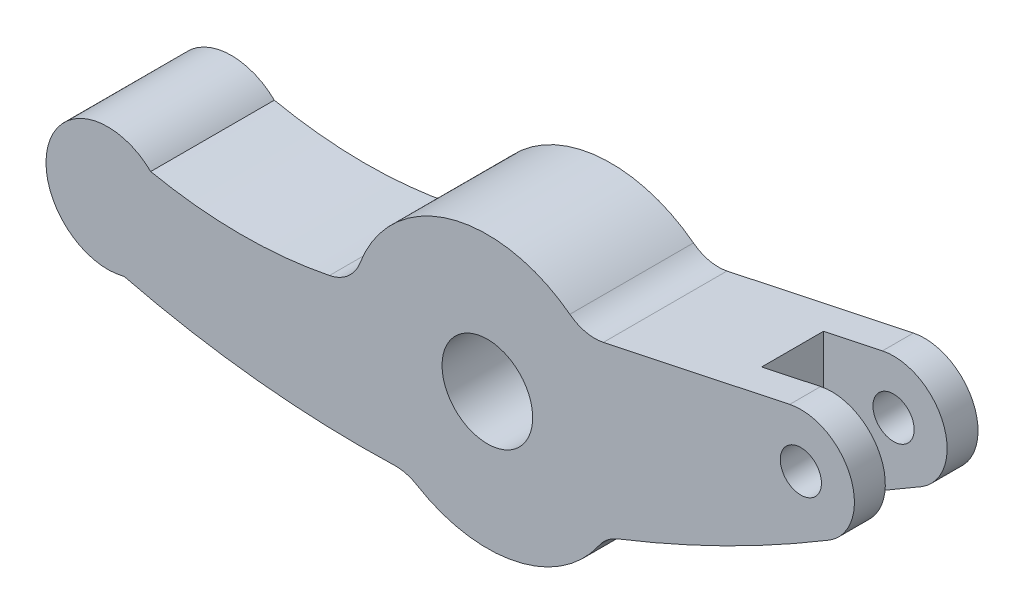
SolidWorks part; units mm, degrees
ref_plane "Front Plane" through (0, 0, 0) normal (0, 0, 1) x (1, 0, 0)
ref_plane "Top Plane" through (0, 0, 0) normal (0, 1, 0) x (1, 0, 0)
ref_plane "Right Plane" through (0, 0, 0) normal (1, 0, 0) x (0, 0, -1)
sketch "Sketch1" plane through (0, 0, 0) normal (0, 0, 1) x (1, 0, 0)
  line L7 (23.3648, -2.4326) -> (82.7627, 3.0066)
  line L8 (23.3729, -8.3627) -> (82.7596, -3.0293)
  arc A14 (23.3648, -2.4326) -> (23.3729, -8.3627) centre (8.6648, -5.4177) ccw
  arc A16 (82.7596, -3.0293) -> (82.7627, 3.0066) centre (100.5064, -0.0205) ccw
extrude "Boss-Extrude1" add sketch "Sketch1" along normal blind 10
sketch "Sketch7" plane through (0, 0, 0) normal (0, 0, -1) x (-1, 0, 0)
  circle A0 centre (-100.78, 0) radius 8
extrude "Cut-Extrude2" cut sketch "Sketch7" against normal blind 10
sketch "Sketch8" plane through (0, 0, 10) normal (0, 0, 1) x (1, 0, 0)
  circle A0 centre (8.6648, -5.4177) radius 6
extrude "Cut-Extrude3" cut sketch "Sketch8" against normal blind 14
sketch "Sketch17" plane through (0, 0, 0) normal (0, 0, -1) x (-1, 0, 0)
  line L1 (-115.8122, 9.3934) -> (-161.8976, 22.2751)
  line L2 (-118.4017, 1.9179) -> (-164.5896, 12.6443)
  arc A0 (-161.8976, 22.2751) -> (-164.5896, 12.6443) centre (-176.8637, 21.2668) ccw
  arc A1 (-118.4017, 1.9179) -> (-115.8122, 9.3934) centre (-100.78, 0) ccw
  circle A2 centre (-100.78, 0) radius 8
  arc A3 (-82.7627, 3.0066) -> (-82.7596, -3.0293) centre (-100.5064, -0.0205) ccw construction
  point P4 (-99.434, 4.8154)
  point P5 (-175.5177, 26.0822)
  point P6 (-102.126, -4.8154)
  point P7 (-178.2097, 16.4513)
extrude "Boss-Extrude2" add sketch "Sketch17" against normal blind 10
sketch "Sketch18" plane through (0, 0, 0) normal (0, 0, -1) x (-1, 0, 0)
  circle A0 centre (-176.8637, 21.2668) radius 6
extrude "Cut-Extrude10" cut sketch "Sketch18" against normal blind 10
sketch "Sketch20" plane through (0, 0, 10) normal (0, 0, 1) x (1, 0, 0)
  circle A0 centre (176.8637, 21.2668) radius 15
sketch "Sketch21" plane through (0, 0, 10) normal (0, 0, 1) x (1, 0, 0)
  circle A0 centre (8.6648, -5.4177) radius 15
sketch "Sketch22" plane through (0, 0, 10) normal (0, 0, 1) x (1, 0, 0)
  circle A0 centre (8.6648, -5.4177) radius 13
sketch "Sketch23" plane through (0, 0, 10) normal (0, 0, 1) x (1, 0, 0)
  line L0 (174.169, 33.9844) -> (97.0897, 17.6522)
  line L1 (181.1377, 8.9894) -> (108.1783, -16.4093)
  arc A0 (8.6648, -18.4177) -> (102.3485, -17.9315) centre (54.4178, 191.6593) ccw
  arc A3 (13.0493, 6.8206) -> (92.6784, 16.1882) centre (41.1609, 110.9854) ccw
  arc A6 (181.1377, 8.9894) -> (174.169, 33.9844) centre (176.8637, 21.2668) ccw
  arc A10 (13.0493, 6.8206) -> (8.6648, -18.4177) centre (8.6648, -5.4177) ccw
  arc A11 (102.3485, -17.9315) -> (108.1783, -16.4093) centre (100.78, 0) ccw
  arc A12 (92.6784, 16.1882) -> (97.0897, 17.6522) centre (100.5064, -0.0205) cw
extrude "Boss-Extrude3" add sketch "Sketch23" along normal blind 10
sketch "Sketch25" plane through (0, 0, 10) normal (0, 0, -1) x (-1, 0, 0)
  circle A0 centre (-8.6648, -5.4177) radius 5
extrude "Cut-Extrude11" cut sketch "Sketch25" against normal blind 20
sketch "Sketch26" plane through (0, 0, 20) normal (0, 0, 1) x (1, 0, 0)
  circle A0 centre (8.6648, -5.4177) radius 8.5
sketch "Sketch29" plane through (0, 0, 10) normal (0, 0, -1) x (-1, 0, 0)
  circle A0 centre (-176.8637, 21.2668) radius 5
extrude "Cut-Extrude12" cut sketch "Sketch29" against normal blind 10
sketch "Sketch30" plane through (0, 0, 0) normal (0, 0, -1) x (-1, 0, 0)
  line L2 (-181.1377, 8.9894) -> (-108.1783, -16.4093)
  line L3 (-97.0897, 17.6522) -> (-174.169, 33.9844)
  line L4 (-181.1377, 8.9894) -> (-108.1783, -16.4093)
  line L5 (-97.0897, 17.6522) -> (-174.169, 33.9844)
  arc A6 (-8.6648, -18.4177) -> (-13.0493, 6.8206) centre (-8.6648, -5.4177) ccw
  arc A7 (-102.3485, -17.9315) -> (-8.6648, -18.4177) centre (-54.4178, 191.6593) ccw
  arc A8 (-108.1783, -16.4093) -> (-102.3485, -17.9315) centre (-100.78, 0) ccw
  arc A9 (-174.169, 33.9844) -> (-181.1377, 8.9894) centre (-176.8637, 21.2668) ccw
  arc A10 (-92.6784, 16.1882) -> (-97.0897, 17.6522) centre (-100.5064, -0.0205) ccw
  arc A11 (-92.6784, 16.1882) -> (-13.0493, 6.8206) centre (-41.1609, 110.9854) ccw
  arc A12 (-8.6648, -18.4177) -> (-13.0493, 6.8206) centre (-8.6648, -5.4177) ccw
  arc A13 (-102.3485, -17.9315) -> (-8.6648, -18.4177) centre (-54.4178, 191.6593) ccw
  arc A14 (-108.1783, -16.4093) -> (-102.3485, -17.9315) centre (-100.78, 0) ccw
  arc A15 (-174.169, 33.9844) -> (-181.1377, 8.9894) centre (-176.8637, 21.2668) ccw
  arc A16 (-92.6784, 16.1882) -> (-97.0897, 17.6522) centre (-100.5064, -0.0205) ccw
  arc A17 (-92.6784, 16.1882) -> (-13.0493, 6.8206) centre (-41.1609, 110.9854) ccw
  dimension "D1" = 0
sketch "Sketch31" plane through (0, 0, 10) normal (0, 0, -1) x (-1, 0, 0)
  circle A0 centre (-100.78, 0) radius 11
extrude "Cut-Extrude13" cut sketch "Sketch31" against normal blind 10
extrude "Boss-Extrude5" add sketch "Sketch30" along normal blind 10 and the other way blind 10 contours L5 A15 L4 A14 A13 A12 A17 A16
sketch "Sketch32" plane through (0, 0, 10) normal (0, 0, 1) x (1, 0, 0)
  circle A0 centre (8.6648, -5.4177) radius 5
  circle A1 centre (100.78, 0) radius 11
  circle A2 centre (176.8637, 21.2668) radius 5
extrude "Cut-Extrude14" cut sketch "Sketch32" against normal blind 20
ref_plane "Plane1" through (0, 0, -2.5) normal (0, 0, -1) x (-1, 0, 0)
sketch "Sketch33" plane through (0, 0, -2.5) normal (0, 0, -1) x (-1, 0, 0)
  line L1 (-25.6648, -5.4177) -> (-25.6648, -33.5873)
  line L2 (-25.6648, -33.5873) -> (16.718, -33.5873)
  line L3 (16.718, -33.5873) -> (16.718, 17.6907)
  line L4 (16.718, 17.6907) -> (-25.6648, 17.6907)
  line L5 (-25.6648, 17.6907) -> (-25.6648, -5.4177)
  line L6 (-159.8637, -3.5732) -> (-159.8637, 44.7912)
  line L7 (-159.8637, -3.5732) -> (-203.6907, -3.5732)
  line L8 (-203.6907, -3.5732) -> (-203.6907, 44.7912)
  line L9 (-203.6907, 44.7912) -> (-159.8637, 44.7912)
extrude "Cut-Extrude15" cut sketch "Sketch33" against normal blind 15
sketch "Sketch36" plane through (0, 0, 20) normal (0, 0, 1) x (1, 0, 0)
  circle A0 centre (139.1279, 11.3772) radius 4
sketch "Sketch37" plane through (0, 0, 20) normal (0, 0, 1) x (1, 0, 0)
  circle A0 centre (8.6648, -5.4177) radius 15
sketch "Sketch38" plane through (0, 0, -10) normal (0, 0, -1) x (-1, 0, 0)
  line L3 (-183.9213, 10.3494) -> (-165.5775, 5.1601)
  line L4 (-165.5775, 5.1601) -> (-95.9299, -17.1103)
  line L5 (-95.9299, -17.1103) -> (-5.6959, -18.0741)
  arc A0 (-111.0892, -22.7754) -> (-100.78, -25) centre (-100.78, 0) ccw
  arc A3 (-174.169, 33.9844) -> (-181.1377, 8.9894) centre (-176.8637, 21.2668) ccw construction
  arc A5 (-5.6959, -18.0741) -> (-100.78, -25) centre (-70.4038, 214.1305) cw
  arc A6 (-183.9213, 10.3494) -> (-111.0892, -22.7754) centre (-6.8528, 303.0422) ccw
extrude "Boss-Extrude7" add sketch "Sketch38" against normal up to surface (30 mm away)
sketch "Sketch39" plane through (0, 0, 0) normal (0, 1, 0) x (1, 0, 0)
  line L0 (-4.3352, 2.5) -> (25.6648, 2.5)
  line L1 (25.6648, 2.5) -> (25.6648, -12.5)
  line L2 (25.6648, -12.5) -> (-5.8603, -12.5)
  line L3 (-5.8603, -12.5) -> (-4.3352, 2.5)
  line L4 (159.8637, 2.5) -> (191.0122, 2.5)
  line L5 (191.0122, 2.5) -> (191.0122, -12.5)
  line L6 (191.0122, -12.5) -> (159.8637, -12.5)
  line L7 (159.8637, -12.5) -> (159.8637, 2.5)
extrude "Cut-Extrude16" cut sketch "Sketch39" against normal blind 62 and the other way blind 66
sketch "Sketch40" plane through (0, 0, -10) normal (0, 0, -1) x (-1, 0, 0)
  circle A0 centre (-139.1279, 11.3772) radius 4
extrude "Cut-Extrude18" cut sketch "Sketch40" against normal blind 15 contours A0
sketch "Sketch41" plane through (0, 0, -10) normal (0, 0, -1) x (-1, 0, 0)
  circle A0 centre (-100.78, 0) radius 33
  circle A1 centre (-100.78, 0) radius 11
extrude "Boss-Extrude8" add sketch "Sketch41" against normal up to surface (30 mm away) contours A0 | A1 up to face at (109.9732, 2.7192, 20)
fillet "Fillet1" radius 10 4 edges at (68.447, 6.6013, 5) (124.0782, 23.3708, 5) (81.3493, -26.673, 5) (129.4653, -16.3142, 5)
ref_plane "Plane2" through (0, 0, 18.5) normal (0, 0, 1) x (1, 0, 0)
ref_plane "Plane3" through (0, 0, -8.5) normal (0, 0, -1) x (-1, 0, 0)
sketch "Sketch42" plane through (0, 0, -10) normal (0, 0, -1) x (-1, 0, 0)
  line L0 (-62.4634, 5.2179) -> (-78.1975, -26.7956)
  arc A0 (-12.6076, -19.8902) -> (-19.0791, 5.3779) centre (-8.6648, -5.4177) ccw
  arc A1 (-78.1975, -26.7956) -> (-5.6959, -18.0741) centre (-70.4038, 214.1305) ccw construction
  arc A2 (-62.4634, 5.2179) -> (-13.0493, 6.8206) centre (-41.1609, 110.9854) ccw construction
  arc A3 (-78.1975, -26.7956) -> (-12.6076, -19.8902) centre (-70.4038, 214.1305) ccw
  arc A4 (-62.4634, 5.2179) -> (-19.0791, 5.3779) centre (-41.1609, 110.9854) ccw
  dimension "D1" = 30
extrude "Boss-Extrude9" add sketch "Sketch42" against normal up to surface (30 mm away) up to face at (106.1059, 1.7833, 20)
